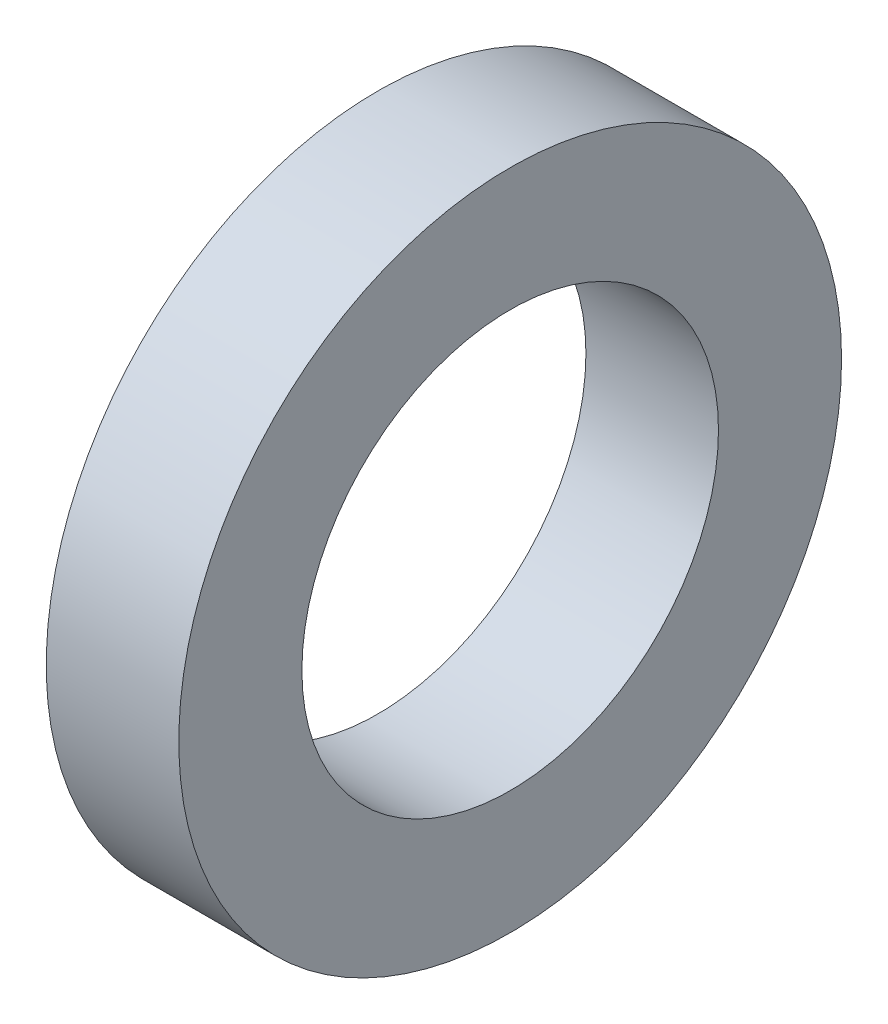
from build123d import *

# Parameters (mm, degrees)
SKETCH_1_R      = 17.5
SKETCH_1_R_2    = 11
EXTRUDE_1_DEPTH = 7


with BuildPart() as part:
    # 草图1 → 凸台-拉伸1 (new body)
    with BuildSketch(Plane(origin=(0, 0, 0), x_dir=(0, 0, -1), z_dir=(1, 0, 0))):
        Circle(SKETCH_1_R)
        Circle(SKETCH_1_R_2, mode=Mode.SUBTRACT)
    extrude(amount=EXTRUDE_1_DEPTH)


solid = part.part
